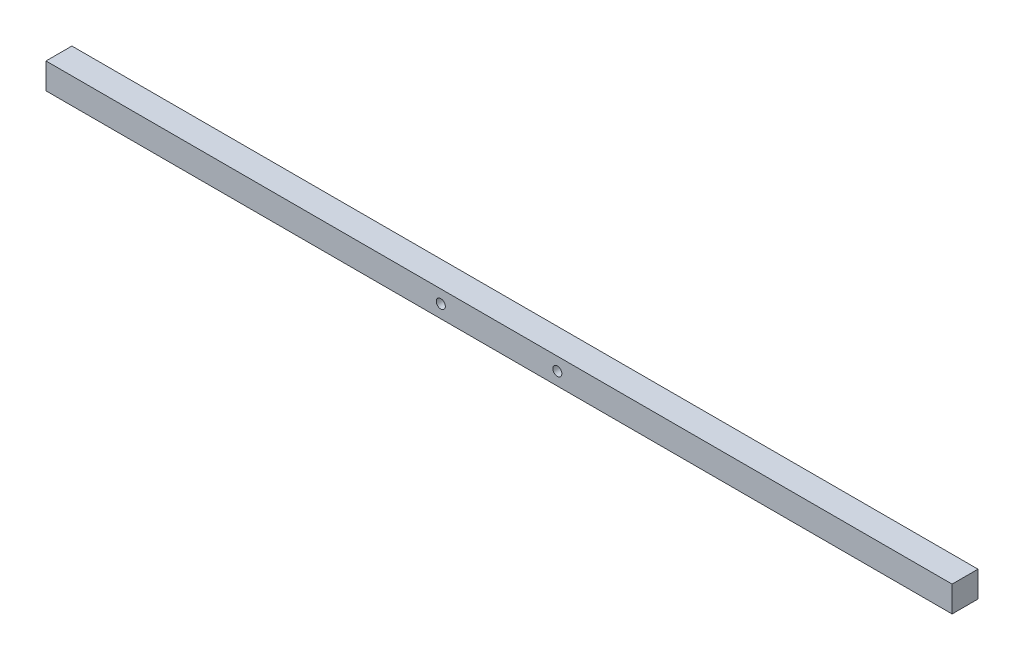
SolidWorks part; units mm, degrees
material "1Cr18Ni9"
ref_plane "前视基准面" through (0, 0, 0) normal (0, 0, 1) x (1, 0, 0)
ref_plane "上视基准面" through (0, 0, 0) normal (0, 1, 0) x (1, 0, 0)
ref_plane "右视基准面" through (0, 0, 0) normal (1, 0, 0) x (0, 0, -1)
sketch "草图1" plane through (0, 0, 0) normal (1, 0, 0) x (0, 0, -1)
  line L1 (-10, 10) -> (10, 10)
  line L2 (-10, 10) -> (-10, -10)
  line L3 (-10, -10) -> (10, -10)
  line L4 (10, 10) -> (10, -10)
  line L5 (-10, 10) -> (10, -10) construction
  line L6 (-10, -10) -> (10, 10) construction
  point P0 (0, 0)
  dimension "D1" = 20
  dimension "D2" = 20
extrude "凸台-拉伸1" add sketch "草图1" along normal mid plane 700
sketch "草图2" plane through (0, 0, 10) normal (0, 0, 1) x (1, 0, 0)
  line L0 (0, 79.3055) -> (0, -93.857) construction
  line L1 (350, 10) -> (-350, 10) construction
  circle A0 centre (-45, 0) radius 3.5
  circle A1 centre (45, 0) radius 3.5
  dimension "D1" = 7
  dimension "D2" = 90
  dimension "D3" = 45
  dimension "D4" = 10
extrude "切除-拉伸1" cut sketch "草图2" against normal blind 700
